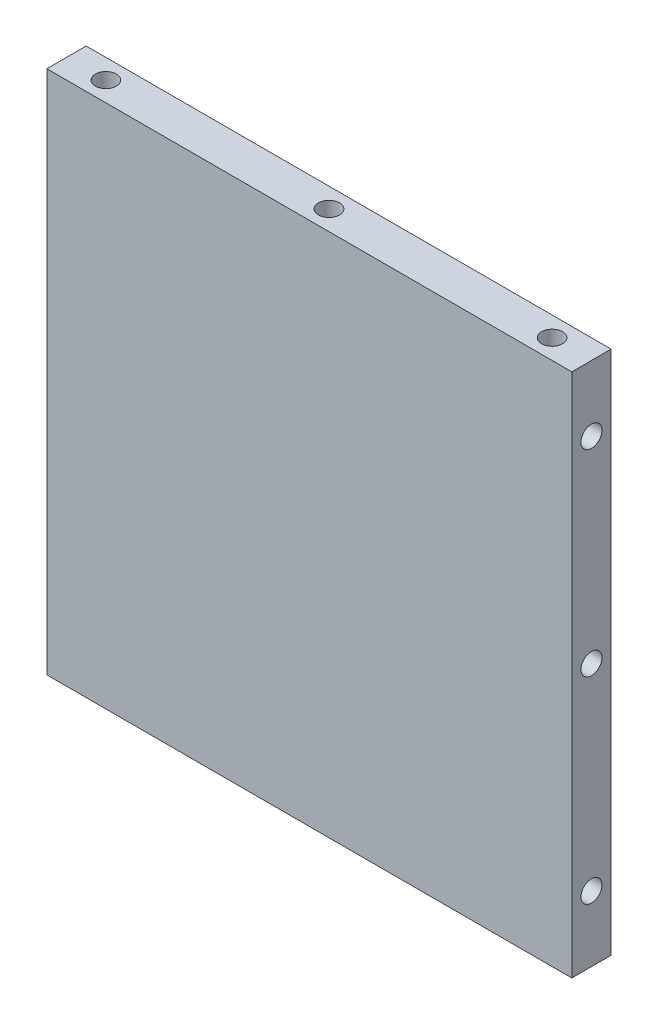
SolidWorks part; units mm, degrees
ref_plane "Front Plane" through (0, 0, 0) normal (0, 0, 1) x (1, 0, 0)
ref_plane "Top Plane" through (0, 0, 0) normal (0, 1, 0) x (1, 0, 0)
ref_plane "Right Plane" through (0, 0, 0) normal (1, 0, 0) x (0, 0, -1)
sketch "Sketch1" plane through (0, 0, 0) normal (0, 0, 1) x (1, 0, 0)
  line L1 (100, -100) -> (-100, -100)
  line L2 (100, -100) -> (100, 100)
  line L3 (100, 100) -> (-100, 100)
  line L4 (-100, -100) -> (-100, 100)
  line L5 (100, -100) -> (-100, 100) construction
  line L6 (100, 100) -> (-100, -100) construction
  point P1 (0, 0)
  dimension "D1" = 200
  dimension "D2" = 200
extrude "Boss-Extrude1" add sketch "Sketch1" along normal blind 15
sketch "Sketch2" plane through (100, 0, 0) normal (1, 0, 0) x (0, 0, -1)
  line L0 (0, 0) -> (-32.3248, 0) construction
  line L1 (-7.5, 100) -> (-7.5, -100) construction
  line L2 (-15, 100) -> (0, 100) construction
  line L3 (-15, -100) -> (0, -100) construction
  circle A0 centre (-7.5, 0) radius 4
  dimension "D1" = 8
extrude "Cut-Extrude1" cut sketch "Sketch2" against normal blind 25
pattern_linear "LPattern1" count 2 spacing 75 along (0, -1, 0) of "Cut-Extrude1"
mirror "Mirror1" about plane through (0, 0, 0) normal (0, 1, 0) of "LPattern1", "Cut-Extrude1"
mirror "Mirror2" about plane through (0, 0, 0) normal (1, 0, 0) of "Mirror1", "LPattern1", "Cut-Extrude1"
sketch "Sketch3" plane through (0, 100, 0) normal (0, 1, 0) x (1, 0, 0)
  circle A0 centre (0, -7.5) radius 4
  dimension "D1" = 8
extrude "Cut-Extrude2" cut sketch "Sketch3" against normal blind 25
pattern_linear "LPattern2" count 2 spacing 85 along (1, 0, 0) of "Cut-Extrude2"
mirror "Mirror3" about plane through (0, 0, 0) normal (1, 0, 0) of "LPattern2", "Cut-Extrude2"
mirror "Mirror4" about plane through (0, 0, 0) normal (0, 1, 0) of "Mirror3", "LPattern2", "Cut-Extrude2"
